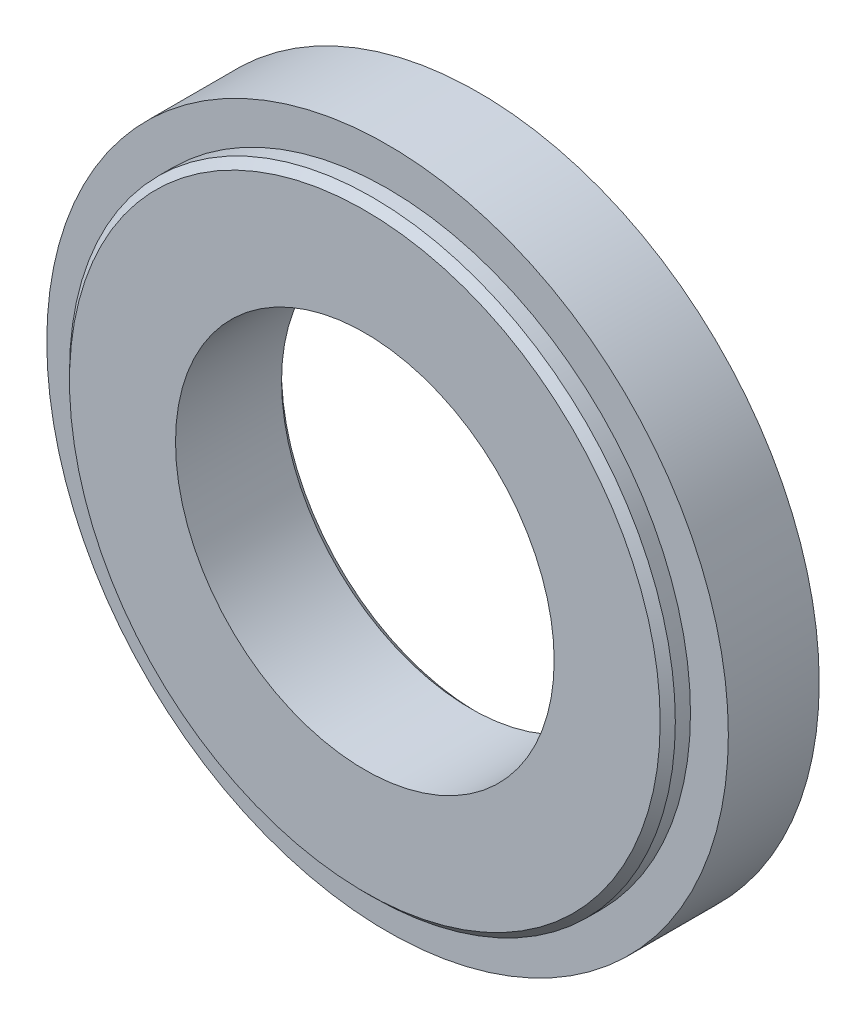
from build123d import *

# Parameters (mm, degrees)
SKETCH1_R           = 45
SKETCH1_R_2         = 25
BOSS_EXTRUDE1_DEPTH = 15
CUT_EXTRUDE1_START  = -3
SKETCH2_R           = 45
SKETCH2_R_2         = 40
CUT_EXTRUDE1_DEPTH  = 3
SKETCH3_R           = 2
CUT_EXTRUDE2_DEPTH  = 11
CHAMFER1_SIZE       = 1


with BuildPart() as part:
    # Sketch1 → Boss-Extrude1 (new body)
    with BuildSketch(Plane.XY):
        Circle(SKETCH1_R)
        Circle(SKETCH1_R_2, mode=Mode.SUBTRACT)
    extrude(amount=BOSS_EXTRUDE1_DEPTH)

    # Sketch2 → Cut-Extrude1 (cut)
    with BuildSketch(Plane.XY.offset(15).offset(CUT_EXTRUDE1_START)):
        Circle(SKETCH2_R)
        Circle(SKETCH2_R_2, mode=Mode.SUBTRACT)
    extrude(amount=CUT_EXTRUDE1_DEPTH, mode=Mode.SUBTRACT)

    # Sketch3 → Cut-Extrude2 (cut)
    with BuildSketch(Plane(origin=(0, 0, 0), x_dir=(-1, 0, 0), z_dir=(0, 0, -1))):
        with Locations((0, 36.5)):
            Circle(SKETCH3_R)
        with Locations((31.609927238, 18.25)):
            Circle(SKETCH3_R)
        with Locations((31.609927238, -18.25)):
            Circle(SKETCH3_R)
        with Locations((0, -36.5)):
            Circle(SKETCH3_R)
        with Locations((-31.609927238, -18.25)):
            Circle(SKETCH3_R)
        with Locations((-31.609927238, 18.25)):
            Circle(SKETCH3_R)
    extrude(amount=-CUT_EXTRUDE2_DEPTH, mode=Mode.SUBTRACT)

    # Chamfer1
    chamfer1_edges = [part.edges().sort_by_distance(p)[0] for p in [
        (-40, 0, 15),
        (-25, 0, 0),
    ]]
    chamfer(chamfer1_edges, length=CHAMFER1_SIZE)


solid = part.part
